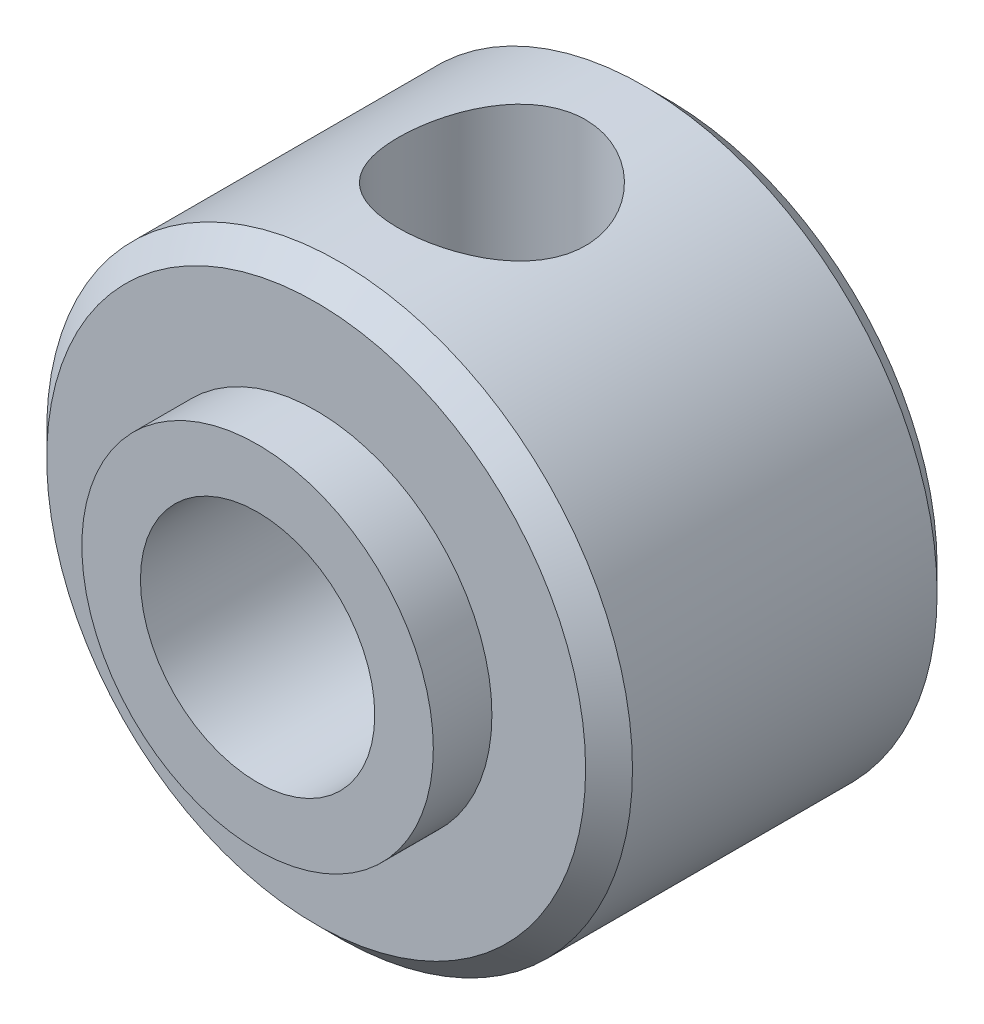
SolidWorks part; units mm, degrees
ref_plane "Front Plane" through (0, 0, 0) normal (0, 0, 1) x (1, 0, 0)
ref_plane "Top Plane" through (0, 0, 0) normal (0, 1, 0) x (1, 0, 0)
ref_plane "Right Plane" through (0, 0, 0) normal (1, 0, 0) x (0, 0, -1)
sketch "Sketch1" plane through (0, 0, 0) normal (0, 0, 1) x (1, 0, 0)
  circle A0 centre (0, 0) radius 2.5
  circle A1 centre (0, 0) radius 1
  dimension "D1" = 2
  dimension "D2" = 5
extrude "Boss-Extrude1" add sketch "Sketch1" along normal mid plane 3
sketch "Sketch2" plane through (0, 0, 1.5) normal (0, 0, 1) x (1, 0, 0)
  circle A0 centre (0, 0) radius 1 construction
  circle A1 centre (0, 0) radius 1
  circle A2 centre (0, 0) radius 1.5
  dimension "D1" = 3
extrude "Boss-Extrude2" add sketch "Sketch2" along normal blind 0.5
hole_wizard "M2 Tapped Hole1" positions "Sketch4" profile "Sketch3" tap size "M2" standard "Gb"
sketch "Sketch4" plane through (0, 0, 0) normal (0, 1, 0) x (1, 0, 0)
  point P0 (0, 0)
sketch "Sketch3" plane through (0, 0, 0) normal (1, 0, 0) x (0, 0, -1)
  line L0 (0, 0) -> (0, 2.5)
  line L1 (0, 2.5) -> (0.8, 2.5)
  line L2 (0.8, 2.5) -> (0.8, 0)
  line L5 (0.8, 0) -> (0, 0)
  line L11 (0, -6.35) -> (0, 107.95) construction
  dimension "通孔螺纹孔钻头直径" = 1.6
  dimension "通孔螺纹孔钻头深度" = 2.5
cosmetic thread "Hole Thread1" parameters "D2"=2
chamfer "Chamfer1" distance 0.2 angle 45 2 edges at (2.5, 0, -1.5) (2.5, 0, 1.5)
